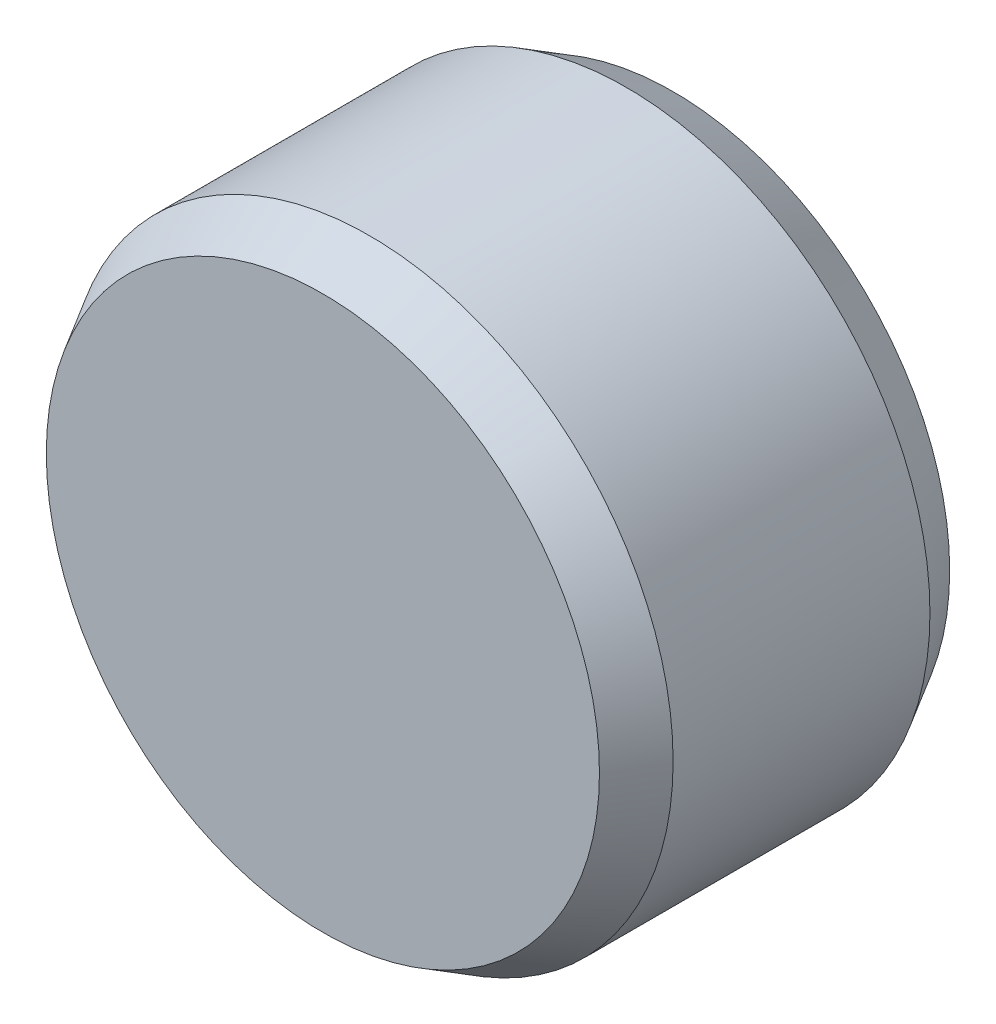
from build123d import *

# Parameters (mm, degrees)
SKETCH_1_R      = 65
EXTRUDE_1_DEPTH = 75
CHAMFER_1_SIZE  = 10
CHAMFER_1_SIZE2 = 5.773502692


with BuildPart() as part:
    # 草图1 → 凸台-拉伸1 (new body)
    with BuildSketch(Plane.XY):
        Circle(SKETCH_1_R)
    extrude(amount=EXTRUDE_1_DEPTH)

    # 倒角1
    chamfer_1_edges = [part.edges().sort_by_distance(p)[0] for p in [
        (-65, 0, 0),
        (-65, 0, 75),
    ]]
    chamfer_1_side = [part.faces().sort_by_distance(p)[0] for p in [
        (-65, 0, 37.5),
    ]]
    chamfer(chamfer_1_edges, length=CHAMFER_1_SIZE, length2=CHAMFER_1_SIZE2, reference=chamfer_1_side[0])


solid = part.part
